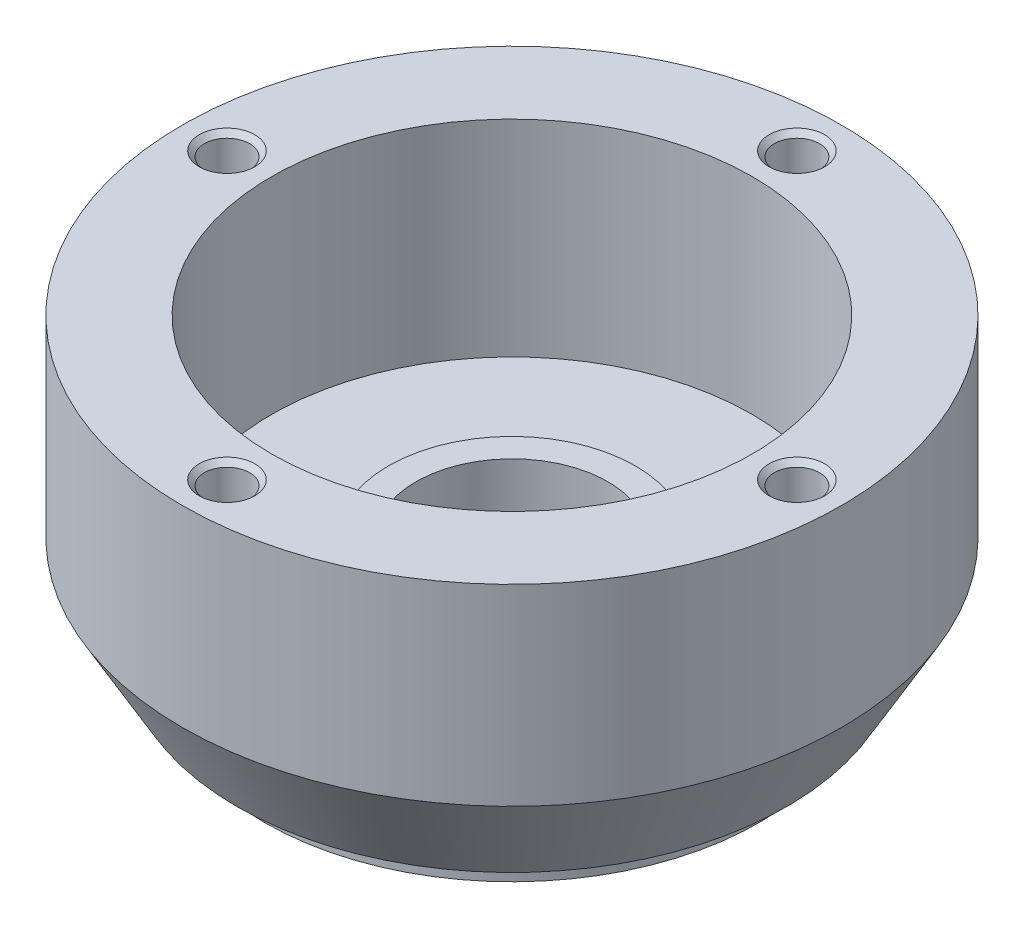
SolidWorks part; units mm, degrees
ref_plane "Front Plane" through (0, 0, 0) normal (0, 0, 1) x (1, 0, 0)
ref_plane "Top Plane" through (0, 0, 0) normal (0, 1, 0) x (1, 0, 0)
ref_plane "Right Plane" through (0, 0, 0) normal (1, 0, 0) x (0, 0, -1)
other "Configuration Table"
sketch "Sketch1" plane through (0, 0, 0) normal (1, 0, 0) x (0, 0, -1)
  line L0 (0, 0) -> (-18, 0)
  line L1 (-18, 0) -> (-18, 2)
  line L2 (-18, 2) -> (-20, 2)
  line L3 (-20, 2) -> (-24, 9)
  line L4 (-24, 9) -> (-24, 23)
  line L5 (-24, 23) -> (0, 23)
  line L6 (0, 23) -> (0, 0) construction
  line L7 (0, 0) -> (0, 23)
  dimension "D1" = 48
  dimension "D2" = 2
  dimension "D3" = 23
  dimension "D4" = 14
  dimension "D5" = 36
  dimension "D6" = 40
revolve "Revolve1" add sketch "Sketch1" angle 360 about L6
sketch "Sketch2" plane through (0, 23, 0) normal (0, 1, 0) x (1, 0, 0)
  circle A0 centre (0, 0) radius 17.5
  dimension "D1" = 35
extrude "Cut-Extrude1" cut sketch "Sketch2" against normal blind 15
sketch "Sketch3" plane through (0, 8, 0) normal (0, 1, 0) x (1, 0, 0)
  circle A0 centre (0, 0) radius 9
  dimension "D1" = 18
extrude "Boss-Extrude1" add sketch "Sketch3" along normal blind 1
sketch "Sketch4" plane through (0, 9, 0) normal (0, 1, 0) x (1, 0, 0)
  circle A0 centre (0, 0) radius 7
  dimension "D1" = 14
extrude "Cut-Extrude2" cut sketch "Sketch4" against normal through all
sketch "Sketch5" plane through (0, 0, 0) normal (0, -1, 0) x (1, 0, 0)
  line L0 (0, 0) -> (0, 14) construction
  circle A0 centre (0, 14) radius 2
  dimension "D1" = 4
  dimension "D2" = 14
extrude "Cut-Extrude3" cut sketch "Sketch5" against normal blind 4
sketch "Sketch6" plane through (0, 0, 0) normal (0, 0, 1) x (1, 0, 0)
  line L0 (-14, 0) -> (-14, 1) construction
  line L1 (-18, 0) -> (18, 0) construction
  line L2 (-16, 0) -> (-14, 0)
  line L3 (-14, 0) -> (-14, 1)
  arc A0 (-14, 1) -> (-16, 0) centre (-13.852, -1.7961) ccw
  dimension "D1" = 2.8
  dimension "D2" = 14
  dimension "D3" = 1
  dimension "D4" = 2
revolve "Cut-Revolve1" cut sketch "Sketch6" angle 360 about L0
pattern_circular "CirPattern1" count 8 over 360 about axis through (0, 0, 0) along (0, 1, 0) skipping 2, 6 of "Cut-Revolve1"
hole_wizard "M4 Tapped Hole1" positions "Sketch7" profile "Sketch8" tap size "M4" standard "GB"
sketch "Sketch7" plane through (0, 23, 0) normal (0, 1, 0) x (1, 0, 0)
  line L0 (0, 0) -> (0, 20.75) construction
  point P0 (0, 20.75)
  dimension "D1" = 20.75
sketch "Sketch8" plane through (0, 23, -20.75) normal (1, 0, 0) x (0, 0, 1)
  line L0 (0, 0) -> (0, 8.9914)
  line L1 (0, 8.9914) -> (1.65, 8)
  line L2 (1.65, 8) -> (1.65, 0.375)
  line L3 (1.65, 0.375) -> (2.025, 0)
  line L5 (2.025, 0) -> (0, 0)
  line L6 (-1.65, 0.375) -> (-2.025, 0) construction
  line L10 (0, 8.9914) -> (-1.65, 8) construction
  line L11 (0, -6.35) -> (0, 107.95) construction
  dimension "螺纹孔钻头直径" = 3.3
  dimension "螺纹孔钻头深度" = 8
  dimension "近端锥形沉头孔直径" = 4.05
  dimension "近端锥形沉头孔角度" = 90
  dimension "导头角度" = 118
cosmetic thread "hole thread 1" parameters "D1"=8, "D2"=4
pattern_circular "CirPattern2" count 4 over 360 about axis through (0, 0, 0) along (0, 1, 0) of "M4 Tapped Hole1"
chamfer "Chamfer1" distance 0.5 angle 45 1 edges at (0, 0, 7)
